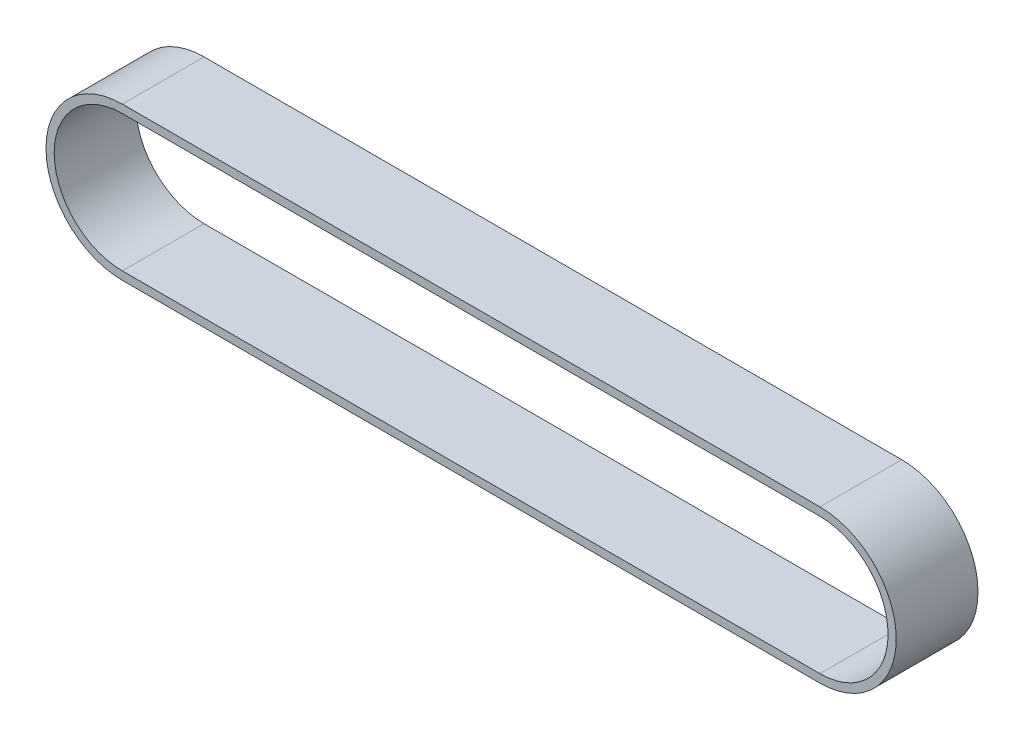
from build123d import *

# Parameters (mm, degrees)
EXTRUDE_1_DEPTH = 30


with BuildPart() as part:
    # 草图1 → 拉伸-薄壁1 (new body)
    with BuildSketch(Plane.XY):
        with BuildLine():
            Line((128, -28), (-128, -28))
            ThreePointArc((-128, -28), (-156, 0), (-128, 28))
            Line((-128, 28), (128, 28))
            ThreePointArc((128, 28), (156, 0), (128, -28))
        make_face()
        with BuildLine():
            Line((128, -25), (-128, -25))
            ThreePointArc((-128, -25), (-153, 0), (-128, 25))
            Line((-128, 25), (128, 25))
            ThreePointArc((128, 25), (153, 0), (128, -25))
        make_face(mode=Mode.SUBTRACT)
    extrude(amount=EXTRUDE_1_DEPTH)


solid = part.part
